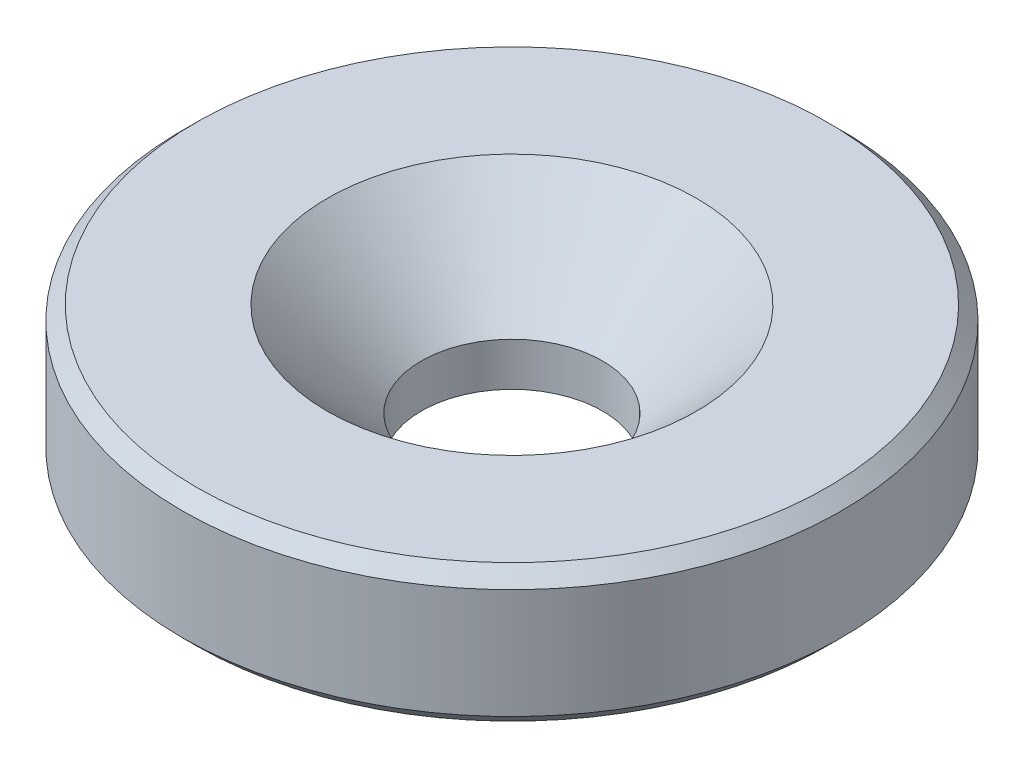
from build123d import *

# Parameters (mm, degrees)
SKETCH_1_R      = 12
EXTRUDE_1_DEPTH = 5
CHAMFER_1_SIZE  = 0.5


with BuildPart() as part:
    # 草图1 → 凸台-拉伸1 (new body)
    with BuildSketch(Plane(origin=(0, 0, 0), x_dir=(1, 0, 0), z_dir=(0, 1, 0))):
        with Locations(Location((0, 0, 0), (0, 0, 270))):
            Circle(SKETCH_1_R)
    extrude(amount=EXTRUDE_1_DEPTH)

    # 草图2 → M6 六角凹锥坑螺钉的锥形沉头孔1 (revolve, cut)
    with BuildSketch(Plane(origin=(0, 5, 0), x_dir=(0, 0, 1), z_dir=(1, 0, 0))):
        Polygon((0, 0), (0, 5), (3.3, 5), (3.3, 3.42), (6.72, 0), align=None)
    revolve(axis=Axis((0, 11.35, 0), (0, -1, 0)), mode=Mode.SUBTRACT)

    # 倒角1
    chamfer_1_edges = [part.edges().sort_by_distance(p)[0] for p in [
        (0, 0, -12),
        (0, 5, -12),
    ]]
    chamfer(chamfer_1_edges, length=CHAMFER_1_SIZE)


solid = part.part
